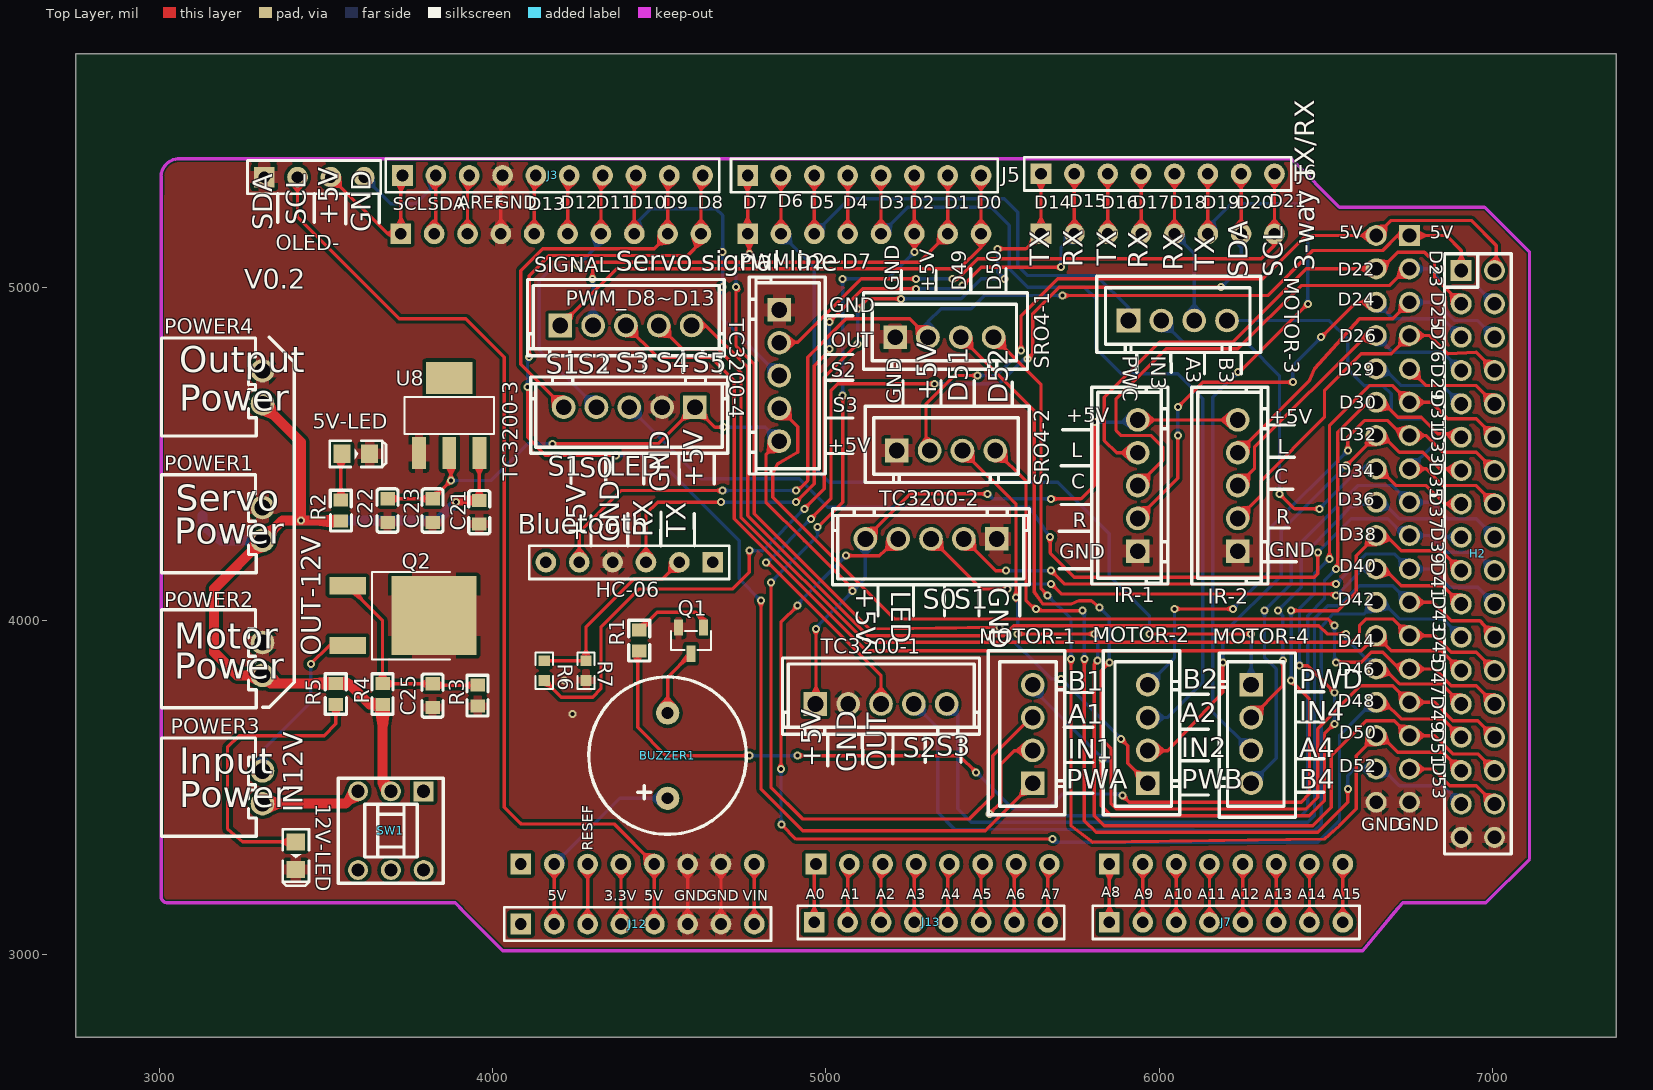
[diagram p0: Top Layer view]
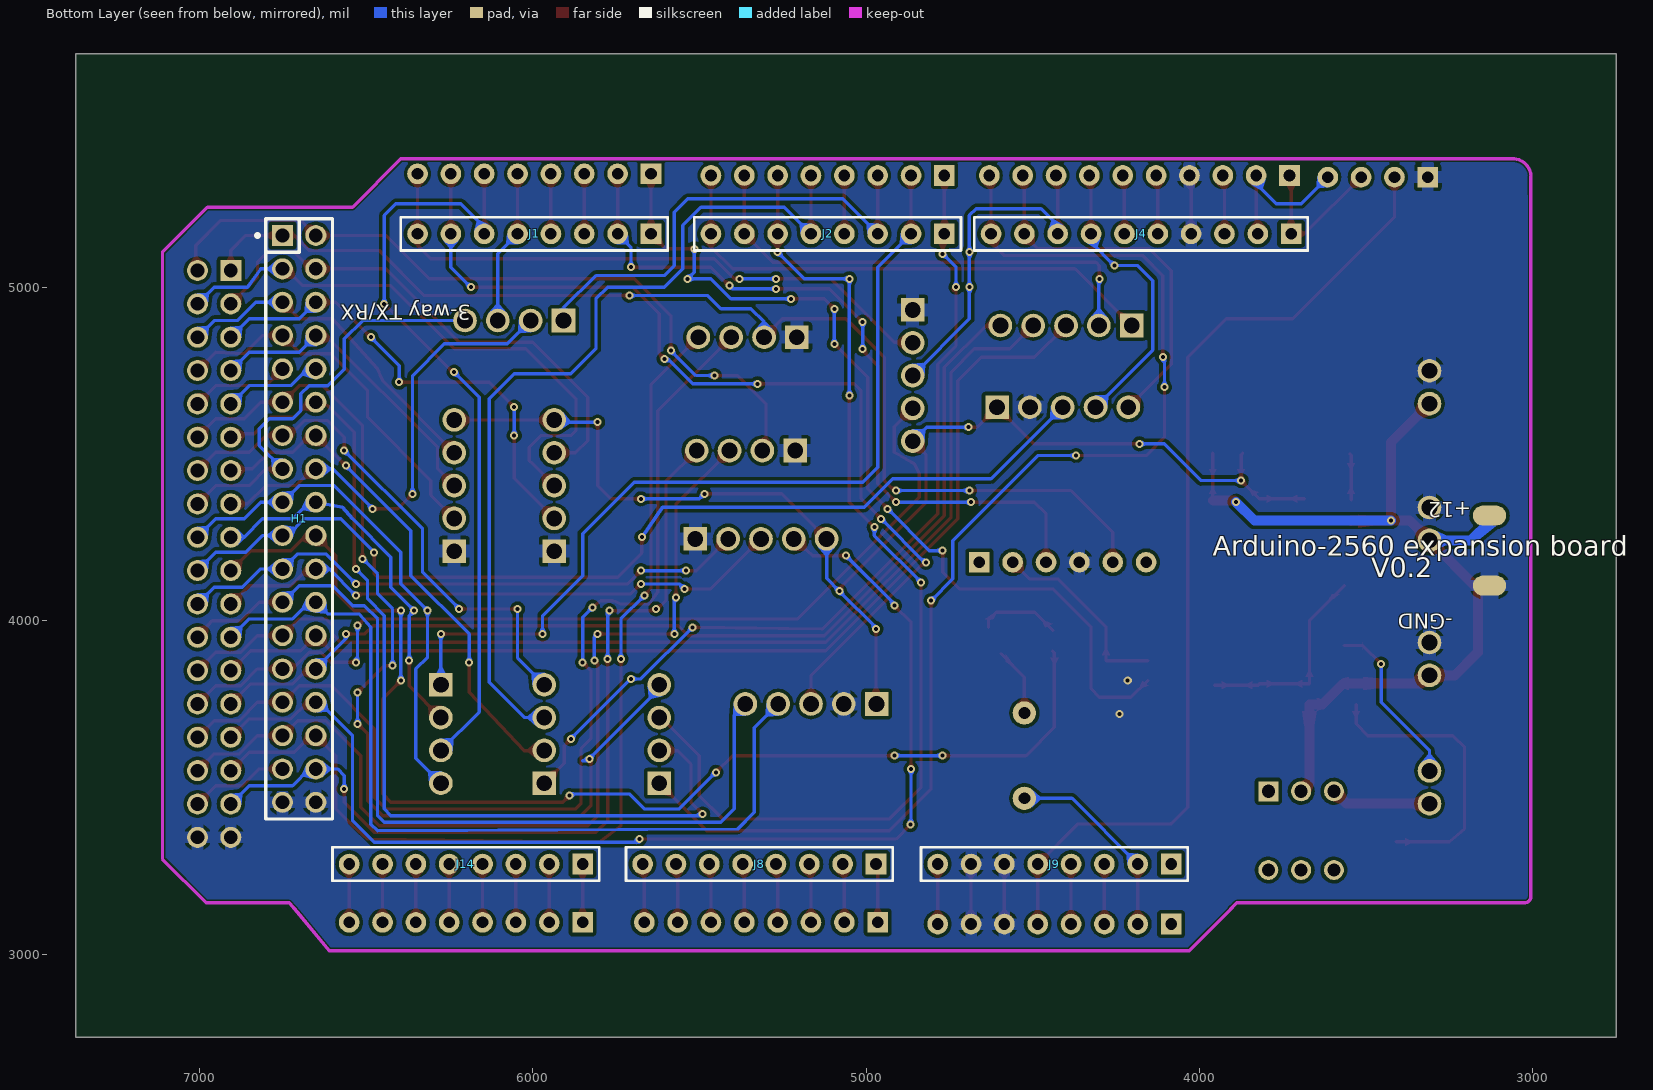
[diagram p1: Bottom Layer view, seen from below]
# Altium PCB MISC49934.pcbdoc (part 1 of 2)
Units mil, origin at the board's own origin, x right, y up, seen from the top; angles counter-clockwise.
Board outline 4620 x 2950 mil, 2 copper layers (Top Layer, Bottom Layer), stack 0 mil thick; 53 components, 145 nets, 295 pads, 118 vias.

## Layer stack, top to bottom
Top Layer: signal copper (thickness not stored)
Bottom Layer: signal copper (thickness not stored)

## Board outline
7370,2750 2750,2750 2750,5700 7370,5700

## Design rules (kind name [scope] priority, off if disabled: settings)
HoleToHoleClearance Default [All] p1 off: gap=0 allowstackedmicrovias=TRUE
HoleToHoleClearance gge14896 [All] p2 off: gap=0 allowstackedmicrovias=TRUE
HoleToHoleClearance gge14902 [All] p3 off: gap=0 allowstackedmicrovias=TRUE
HoleToHoleClearance Common [All] p4: gap=11.8 allowstackedmicrovias=TRUE

## Components (designator, comment, footprint, x,y, rotation, side; value= is the part's Value field where it differs from the comment)
5V-LED "LED-0805_R" LED0805_RED 3590,4500 r0 top
12V-LED "LED-0805_R" LED0805_RED 3410,3295 r270 top
+12 "Pad" 焊盘 3130,4315 r180 bottom
-GND "Pad" 焊盘 3130,4105 r180 bottom
BUZZER1 "GMC1205YA-16R2048" BUZ-TH_BD12.0-P6.50-D0.6-FD 4525,3595 r90 top
C21 "100nf" C0603 3960,4325 r90 top
C22 "100nf" C0603 3685,4330 r90 top
C23 "100nf" C0603 3820,4330 r90 top
C25 "100nf" C0603 3820,3775 r90 top
H1 "X6521WV-2×18H-C30D60" HDR-TH_36P-2.54-V-M-R2-C18-S2.54 6700,4305 r270 bottom locked
H2 "X6521WV-2×18H-C30D60" HDR-TH_36P-2.54-V-M-R2-C18-S2.54 6955,4200 r270 top locked
HC-06 "Bluetooth" HDR-F-2.54_1X6 4460,4175 r180 top
IR-1 "XH-5A_C722874" CONN-TH_XH-5A 5935,4405 r90 top
IR-2 "XH-5A_C722874" CONN-TH_XH-5A 6235,4405 r90 top
J1 "3-way TX/RX" HDR-M-2.54_1X8 6045,5160 r0 bottom locked
J2 "PWM D2~D7" HDR-M-2.54_1X8 5165,5160 r0 bottom locked
J3 "PWM_D8~D13" HDR-M-2.54_1X10#1 4180,5335 r0 top
J4 "PWM_D8~D13" HDR-M-2.54_1X10#2 4175,5160 r0 bottom
J5 "PWM D2~D7" HDR-M-2.54_1X8 5165,5335 r0 top
J6 "3-way TX/RX" HDR-M-2.54_1X8 6045,5340 r0 top
J7 "HDR-M-2.54_1x8" HDR-M-2.54_1X8 6250,3095 r0 top
J8 "HDR-M-2.54_1x8" HDR-M-2.54_1X8 5370,3270 r0 bottom
J9 "HDR-M-2.54_1x8" HDR-M-2.54_1X8 4485,3270 r0 bottom locked
J12 "HDR-M-2.54_1x8" HDR-M-2.54_1X8 4485,3090 r0 top
J13 "HDR-M-2.54_1x8" HDR-M-2.54_1X8 5365,3095 r0 top
J14 "HDR-M-2.54_1x8" HDR-M-2.54_1X8 6250,3270 r0 bottom locked
MOTOR-1 "MOTOR-1" CONN-TH_4P-P2.50_XH-4A 5620,3660 r90 top
MOTOR-2 "MOTOR-2" CONN-TH_4P-P2.50_XH-4A 5965,3660 r90 top
MOTOR-3 "MOTOR-3" CONN-TH_4P-P2.50_XH-4A 6055,4900 r0 top
MOTOR-4 "MOTOR-4" CONN-TH_4P-P2.50_XH-4A 6275,3660 r270 top
OLED- "OLED_" HDR-F-2.54_1X4 3465,5330 r0 top
POWER1 "XH-2AW" CONN-TH_2P-P2.50_XH-2AW 3310,4290 r90 top
POWER2 "XH-2AW" CONN-TH_2P-P2.50_XH-2AW 3310,3885 r90 top
POWER3 "XH-2AW" CONN-TH_2P-P2.50_XH-2AW 3310,3500 r90 top
POWER4 "XH-2AW" CONN-TH_2P-P2.50_XH-2AW 3310,4700 r90 top
Q1 "S8050" SOT-23-3_L2.9-W1.3-P1.90-LS2.4-BR 4595,3940 r90 top
Q2 "KIA50N03A" TO-252-2_L6.6-W6.1-P4.57-LS9.9-TL-CW 3695,4015 r0 top
R1 "10k" R0603#1 4440,3940 r90 top
R2 "200" R0603#1 3545,4330 r270 top
R3 "10K" R0603#1 3955,3775 r90 top
R4 "10k" R0603#1 3670,3780 r90 top
R5 "4.7k" R0603#1 3530,3780 r270 top
R6 "10K" R0603#2 4155,3850 r270 top
R7 "20K" R0603#2 4280,3850 r90 top
SIGNAL "XH-5A_C722874" CONN-TH_XH-5A 4400,4885 r0 top
SRO4-1 "Ultrasonic module" CONN-TH_4P-P2.50_XH-4A 5355,4850 r0 top
SRO4-2 "Ultrasonic module" CONN-TH_4P-P2.50_XH-4A 5360,4510 r0 top
SW1 "XKB8080-Z" SW-TH_6P-L8.0-W8.0-P2.50 3695,3370 r180 top
TC3200-1 "XH-5A_C722874" CONN-TH_XH-5A 5165,3750 r0 top
TC3200-2 "XH-5A_C722874" CONN-TH_XH-5A 5315,4245 r180 top
TC3200-3 "XH-5A_C722874" CONN-TH_XH-5A 4410,4640 r180 top
TC3200-4 "XH-5A_C722874" CONN-TH_XH-5A 4860,4735 r270 top
U8 "AMS1117-5.0" SOT-223_L6.5-W3.5-P2.30-LS7.0-BR 3870,4615 r270 top

## Footprints (in the part's own frame and the unit in brackets; to place one, negate y for a bottom-side part, rotate by r counter-clockwise, add the part's x,y. Pads: shape width x height; smd on the part's side, far side on the other; paste and mask are expansions set on the pad)
BUZ-TH_BD12.0-P6.50-D0.6-FD [mil]
  round 70 hole 35.4: 1(-128,0) 2(128,0)
  silkscreen extent -236,-236 236,236
C0603 [mm]
  rect 1x1.1 smd paste+0 mask+0.102: 1(-0.9,0) 2(0.9,0)
  silkscreen extent -1.65,-0.8 1.65,0.8
CONN-TH_2P-P2.50_XH-2AW [mm]
  round 1.8 hole 1.199: 1(-1.251,0) 2(1.251,0)
  silkscreen extent -3.71,0.48 3.75,7.7
CONN-TH_4P-P2.50_XH-4A [mm]
  rect 1.8x1.8 hole 1.199: 1(-3.75,0)
  round 1.8 hole 1.199: 2(-1.25,0) 3(1.25,0) 4(3.75,0)
  silkscreen extent -6.17,-2.44 6.33,3.38
CONN-TH_XH-5A [mm]
  rect 1.8x1.8 hole 1.2: 1(-5,0)
  round 1.8 hole 1.2: 2(-2.5,0) 3(0,0) 4(2.5,0) 5(5,0)
  silkscreen extent -7.5,-2.3 7.5,3.5
HDR-F-2.54_1X4 [mil]
  rect 62x62 hole 35: 1(-150,0)
  round 62 hole 35: 2(-50,0) 3(50,0) 4(150,0)
  silkscreen extent -200,-50 200,50
HDR-F-2.54_1X6 [mil]
  rect 62x62 hole 35: 1(-200,0)
  round 62 hole 35: 2(-100,0) 3(0,0) 4(100,0) 5(200,0) 6(300,0)
  silkscreen extent -250,-50 350,50
HDR-M-2.54_1X8 [mil]
  rect 62x62 hole 35: 1(-400,0)
  round 62 hole 35: 2(-300,0) 3(-200,0) 4(-100,0) 5(0,0) 6(100,0) 7(200,0) 8(300,0)
  silkscreen extent -450,-50 350,50
HDR-M-2.54_1X10#1 [mil]
  rect 62x62 hole 37.2: 1(-450,0)
  round 62 hole 35: 2(-350,0) 3(-250,0) 4(-150,0) 5(-50,0) 6(50,0) 7(150,0) 8(250,0) 9(350,0) 10(450,0)
  silkscreen extent -500,-50 500,50
HDR-M-2.54_1X10#2 [mil]
  rect 62x62 hole 35: 1(-450,0)
  round 62 hole 35: 2(-350,0) 3(-250,0) 4(-150,0) 5(-50,0) 6(50,0) 7(150,0) 8(250,0) 9(350,0) 10(450,0)
  silkscreen extent -500,-50 500,50
HDR-TH_36P-2.54-V-M-R2-C18-S2.54 [mm]
  rect 1.6x1.6 hole 1.05: 1(-21.59,-1.27)
  round 1.6 hole 1.05: 2(-21.59,1.27) 3(-19.05,-1.27) 4(-19.05,1.27) 5(-16.51,-1.27) 6(-16.51,1.27) 7(-13.97,-1.27) 8(-13.97,1.27) 9(-11.43,-1.27) 10(-11.43,1.27) 11(-8.89,-1.27) 12(-8.89,1.27) 13(-6.35,-1.27) 14(-6.35,1.27) 15(-3.81,-1.27) 16(-3.81,1.27) 17(-1.27,-1.27) 18(-1.27,1.27) 19(1.27,-1.27) 20(1.27,1.27) 21(3.81,-1.27) 22(3.81,1.27) 23(6.35,-1.27) 24(6.35,1.27) 25(8.89,-1.27) 26(8.89,1.27) 27(11.43,-1.27) 28(11.43,1.27) 29(13.97,-1.27) 30(13.97,1.27) 31(16.51,-1.27) 32(16.51,1.27) 33(19.05,-1.27) 34(19.05,1.27) 35(21.59,-1.27) 36(21.59,1.27)
  silkscreen extent -22.86,-3.3 22.86,2.54
LED0805_RED [mil]
  rect 51.2x55.1 smd: 1(-41.35,0) 2(41.35,0)
  silkscreen extent -79,-39 91,39
R0603#1 [mm]
  rect 1x1.1 smd paste+0 mask+0.102: 1(-0.8,0) 2(0.8,0)
  silkscreen extent -1.55,-0.8 1.55,0.81
R0603#2 [mm]
  rect 0.806x0.864 smd paste-100 mask+0.051: 1(-0.753,0) 2(0.753,0)
  silkscreen extent -1.39,-0.66 1.39,0.66
SOT-23-3_L2.9-W1.3-P1.90-LS2.4-BR [mm]
  rect 1.25x0.7 smd: 1(1,-0.95) 2(1,0.95) 3(-1,0)
  silkscreen extent -0.73,-1.53 0.73,1.53
SOT-223_L6.5-W3.5-P2.30-LS7.0-BR [mm]
  rect 2.465x1.05 smd: 1(2.858,-2.3) 2(2.857,0) 3(2.857,2.3)
  rect 2.465x3.54 smd: 4(-2.857,0)
  silkscreen extent -1.4,-3.4 1.4,3.4
SW-TH_6P-L8.0-W8.0-P2.50 [mil]
  rect 60x60 hole 39.37: 1(-98.41,-118.11)
  round 60 hole 39.37: 2(-0.01,-118.11) 3(98.41,-118.11) 4(-98.41,118.11) 5(-0.01,118.11) 6(98.41,118.11)
  silkscreen extent -157,-157 157,157
TO-252-2_L6.6-W6.1-P4.57-LS9.9-TL-CW [mm]
  rect 2.8x1.3 smd: 1(-3.292,2.273) 3(-3.292,-2.273)
  rect 6.5x6 smd: 2(3.292,0)
  silkscreen extent -1.46,-3.35 4.51,3.34
焊盘 [mil]
  oval 100x60 smd paste+0 mask+4: 1(0,0)

## Via types
v1: diameter 24, hole 12, Top Layer to Bottom Layer, 118 vias

## Nets (pads, with @x,y where several pads share a name; then routed paths per layer and width w, separated by ;. In a path a pad name is that pad's centre, name@x,y a point inside that pad or via, vN(x,y) a via of type N, cw(c..) or ccw(c..) an arc to the next point about the centre after c; other vN are vias at no path point)
3.3V: J9.4 J12.4 | length 180
  Top Layer w10: J12.4@4385,3090 J9.4@4385,3270
+5V_1: BUZZER1.1 J9.2 J12.2 | length 601.6
  Top Layer w10: J12.2@4185,3090 J9.2@4185,3270
  Bottom Layer w10: J9.2@4185,3270 4382,3467 BUZZER1.1@4525,3467
+5V_2: J9.5 J12.5 OLED-.2 | length 2964.7
  Top Layer w10: OLED-.2@3415,5330 3415,5210 3720,4905 3920,4905 4035,4790 4035,3440 4075,3400 4085.4,3390 ; 4085,3390 4365,3390 J9.5@4485,3270 J12.5@4485,3090
+5V_3: H1.1 H2.1 HC-06.5 SRO4-1.2 | length 3471.4
  Top Layer w10: HC-06.5@4260,4175 4260,4265 4385,4390 v1(4690,4390) ; v1(4910,4390) 4915,4390 4945,4420 4945,4790 5060,4905 5250.79,4905 SRO4-1.2@5305.79,4850 ; v1(5710,4975) 6325,4975 6460,5110 6670,5110 6715,5155 H1.1@6750,5155 6860,5155 6905,5110 H2.1@6905,5050
  Bottom Layer w10: v1(4690,4390) v1(4910,4390) ; SRO4-1.2@5305.79,4850 5305.79,4895.79 5345,4935 5435,4935 5475,4975 v1(5710,4975)
+5V_4: H1.2 H2.2 SRO4-2.2 | length 2251.9
  Top Layer w10: SRO4-2.2@5310.79,4510 5300,4520.79 5300,4550 5300,4650 5385,4735 v1(5455,4735) ; v1(5585,4810) 5585,4915 5695,5025 6310,5025 6440,5155 H1.2@6650,5155 6695,5200 6935,5200 7010,5125 7010,5055 H2.2@7005,5050
  Bottom Layer w10: v1(5455,4735) 5510,4735 v1(5585,4810)
_AREF: J3.3 J4.3 | length 177.1
  Top Layer w10: J4.3@3925,5160 3925,5330 J3.3@3930,5335
_SCL: J3.1 J4.1 OLED-.3 | length 457.5
  Top Layer w10: OLED-.3@3515,5330 3685,5160 J4.1@3725,5160 3725,5330 J3.1@3730,5335
_SDA: J3.2 J4.2 OLED-.4 | length 478
  Top Layer w10: J4.2@3825,5160 3830,5159.95 J3.2@3830,5335
  Bottom Layer w10: OLED-.4@3615,5330 3695,5250 3770,5250 3830,5310 J3.2@3830,5335
A0: J8.1 J13.1 | length 177.1
  Top Layer w10: J13.1@4965,3095 4965,3265 J8.1@4970,3270
A1: J8.2 J13.2 | length 177.1
  Top Layer w10: J13.2@5065,3095 5065,3265 J8.2@5070,3270
A2: J8.3 J13.3 | length 177.1
  Top Layer w10: J13.3@5165,3095 5165,3265 J8.3@5170,3270
A3: J8.4 J13.4 | length 177.1
  Top Layer w10: J13.4@5265,3095 5265,3265 J8.4@5270,3270
A4: J8.5 J13.5 | length 177.1
  Top Layer w10: J13.5@5365,3095 5365,3265 J8.5@5370,3270
A5: J8.6 J13.6 | length 177.1
  Top Layer w10: J13.6@5465,3095 5465,3265 J8.6@5470,3270
A6: J8.7 J13.7 | length 176.2
  Top Layer w10: J13.7@5565,3095 5565,3260 J8.7@5570,3270
A7: J8.8 J13.8 | length 177.1
  Top Layer w10: J13.8@5665,3095 5665,3265 J8.8@5670,3270
A8: J7.1 J14.1 | length 175
  Top Layer w10: J7.1@5850,3095 J14.1@5850,3270
A9: J7.2 J14.2 | length 175
  Top Layer w10: J7.2@5950,3095 J14.2@5950,3270
A10: J7.3 J14.3 | length 175
  Top Layer w10: J7.3@6050,3095 J14.3@6050,3270
A11: J7.4 J14.4 | length 175
  Top Layer w10: J7.4@6150,3095 J14.4@6150,3270
A12: J7.5 J14.5 | length 175
  Top Layer w10: J7.5@6250,3095 J14.5@6250,3270
A13: J7.6 J14.6 | length 175
  Top Layer w10: J7.6@6350,3095 J14.6@6350,3270
A14: J7.7 J14.7 | length 175
  Top Layer w10: J7.7@6450,3095 J14.7@6450,3270
A15: J7.8 J14.8 | length 175
  Top Layer w10: J7.8@6550,3095 J14.8@6550,3270
D0: J2.8 J5.8 SIGNAL.1 | length 1574.2
  Top Layer w10: SIGNAL.1@4203.1,4885 4373.1,5055 5400,5055 5465,5120 J2.8@5465,5160 J5.8@5465,5335
D1: J2.7 J5.7 SIGNAL.2 | length 1460
  Top Layer w10: v1(4300,5025) 4300,5065 4310,5075 5280,5075 J2.7@5365,5160 J5.7@5365,5335
  Bottom Layer w10: v1(4300,5025) 4301.58,5023.42 SIGNAL.2@4301.58,4885.01
D2: J2.6 J5.6 MOTOR-1.3 | length 3439.4
  Top Layer w10: v1@4835,4120 4835,3500 4930,3405 5430,3405 5500,3475 5500,3594.2 MOTOR-1.3@5620,3714.2 ; v1(4975,4280) 5050,4355 ; v1(5265,5105) J2.6@5265,5160 J5.6@5265,5335 ; 5050,4355 v1(5050,4675) 5050,4355
  Bottom Layer w10: v1(4835,4115) 4975,4255 v1(4975,4280) ; v1(5050,4675) v1(5050,5025) 5185,5025 v1(5265,5105)
D3: J2.5 J5.5 MOTOR-2.3 | length 2634.1
  Top Layer w10: J2.5@5165,5160 J5.5@5165,5335
  Bottom Layer w10: J2.5@5165,5160 5245,5240 5495,5240 5550,5185 5550,5055 5605,5000 5775,5000 5810,4965 5810,4815 5885,4740 6055,4740 6130,4665 6130,3815 6024.21,3709.21 MOTOR-2.3@5965,3709.21
D4: J2.4 J5.4 | length 175
  Top Layer w10: J2.4@5065,5160 J5.4@5065,5335
D5: J2.3 J5.3 MOTOR-3.1 | length 1427.8
  Top Layer w10: J2.3@4965,5160 J5.3@4965,5335
  Bottom Layer w10: J2.3@4965,5160 5070,5265 5535,5265 5575,5225 5575,5065 5605,5035 5810,5035 5907.3,4937.6 MOTOR-3.1@5907.3,4900
D6: J2.2 J5.2 MOTOR-4.1 | length 2691.4
  Top Layer w10: J2.2@4865,5160 J5.2@4865,5335 ; v1(5970,3960) v1(6275,3960)
  Bottom Layer w10: J2.2@4865,5160 4965,5060 4965,4460 5010,4415 5695,4415 5850,4260 5850,4135 5970,4015 v1(5970,3960) ; MOTOR-4.1@6275,3807.65 v1(6275,3960)
D7: J2.1 J5.1 MOTOR-2.1 | length 2603.4
  Top Layer w10: v1(4730,5000) 4730,4825 4785,4768.4 4785,4320 5130,3975 5135,3975 v1(5520,3980) ; J5.1@4765,5335 J2.1@4765,5160 4770,5155 v1(4770,5100) ; v1(5885,3645) 5905,3625 5905,3572.4 MOTOR-2.1@5965,3512.35
  Bottom Layer w10: v1(4730,5000) 4730,5060 v1(4770,5100) ; v1(5520,3980) 5675,3825 v1(5705,3825) v1(5885,3645)
D8: J3.10 J4.10 MOTOR-1.1 | length 3706.7
  Top Layer w10: v1(4105,4700) 4105,4550 4160,4495 v1(4370,4495) ; v1(4110,4790) 4110,5035 4170,5095 4585,5095 4625,5135 J4.10@4625,5160 4625,5330 J3.10@4630,5335 ; v1(4805,4060) 4805,3495 4930,3370 5435,3370 5477.7,3370 MOTOR-1.1@5620,3512.35
  Bottom Layer w10: v1(4105,4700) 4105,4785 v1(4110,4790) ; v1(4370,4495) 4485,4495 4740,4240 4740,4125 v1(4805,4060)
D9: J3.9 J4.9 TC3200-3.5 | length 1128.6
  Top Layer w10: TC3200-3.5@4213.1,4640 4085,4768.2 4085,5050 4150,5115 4485,5115 4525,5155 J4.9@4525,5160 4525,5330 J3.9@4530,5335
D10: J3.8 J4.8 TC3200-4.3 | length 1046.5
  Top Layer w10: J4.8@4425,5160 4425,5330 J3.8@4430,5335
  Bottom Layer w10: J4.8@4425,5160 4425,5185 4475,5235 4670,5235 4690,5215 v1(4690,5105) v1(4690,5000) 4690,4905 TC3200-4.3@4860,4735
D11: J3.7 J4.7 TC3200-3.4 | length 885.8
  Top Layer w10: J4.7@4325,5160 4325,5330 J3.7@4330,5335
  Bottom Layer w10: TC3200-3.4@4311.57,4639.99 4140,4811.57 4140,5020 4185,5065 v1(4255,5065) 4325,5135 J4.7@4325,5160
D12: J3.6 J4.6 | length 177.1
  Top Layer w10: J4.6@4225,5160 4225,5330 J3.6@4230,5335
D13: J3.5 J4.5 | length 177.1
  Top Layer w10: J4.5@4125,5160 4125,5330 J3.5@4130,5335
D14: J1.1 J6.1 R6.2 | length 3580.6
  Top Layer w10: v1(4770,4210) 4770,4145 4720,4095 ; v1(4935,4335) 4995,4395 4995,4730 v1(5095,4830) ; v1(5095,4935) 5125,4965 v1(5225,4965) ; v1(5515,5115) 5600,5115 J1.1@5645,5160 J6.1@5645,5340 ; 4205.3,3770 R6.2@4155,3820.34 4205.3,3770 ; 4205.3,3770 4300,3770 ; 4205.3,3770 4300,3770 ; 4300,3770 4325,3795 ; 4300,3770 4325,3795 ; 4325,3795 4325,3980 ; 4325,3795 4325,3980 ; 4325,3980 4440,4095 ; 4325,3980 4440,4095 ; 4440,4095 4720,4095 ; 4440,4095 4720,4095
  Bottom Layer w10: v1(4770,4210) 4810,4210 v1(4935,4335) ; v1(5095,4830) v1(5095,4935) ; v1(5225,4965) 5405,4965 5465,5025 v1(5535,5025) 5515,5045 v1(5515,5115)
  other v1: 5095,4935
D15: HC-06.3 J1.2 J6.2 | length 2250.8
  Top Layer w10: HC-06.3@4460,4175 4460,4320 4495,4355 v1(4685,4355) ; v1(4910,4355) 4965,4410 4965,4765 5010,4810 v1(5010,4815) ; v1(5010,4895) 5110,4995 v1(5270,4995) ; v1(5410,5005) 5465,5060 v1(5705,5060) ; J1.2@5745,5160 J6.2@5745,5340
  Bottom Layer w10: v1(4685,4355) v1(4910,4355) ; v1(5010,4815) v1(5010,4895) ; v1(5270,4995) 5400,4995 v1(5410,5005) ; v1(5705,5060) 5705,5120 J1.2@5745,5160
D16: J1.3 J6.3 | length 180
  Top Layer w10: J1.3@5845,5160 J6.3@5845,5340
D17: J1.4 J6.4 | length 180
  Top Layer w10: J1.4@5945,5160 J6.4@5945,5340
D18: J1.5 J6.5 MOTOR-3.3 | length 464.5
  Top Layer w10: J1.5@6045,5160 J6.5@6045,5340
  Bottom Layer w10: J1.5@6045,5160 6104.21,5100.79 MOTOR-3.3@6104.21,4900
D19: J1.6 J6.6 MOTOR-4.3 | length 2323.4
  Top Layer w10: J1.6@6145,5160 J6.6@6145,5340 ; v1(6235,4745) 6240,4745 v1(6445,4950) v1@6450,4955
  Bottom Layer w10: J1.6@6145,5160 6145,5180 6215,5250 6410,5250 6440,5220 6445,5215 v1(6445,4950) ; v1(6235,4745) 6160,4670 6160,4555.27 6160,3725.79 MOTOR-4.3@6275,3610.79
D20: J1.7 J6.7 TC3200-1.3 | length 3560.2
  Top Layer w10: v1(4820,4175) 4825,4175 5165,3835 TC3200-1.3@5165,3750 ; v1(5325,4710) 5035,4710 5015,4690 ; 5695,4995 5620,4920 ; v1(6185,5000) 5700,5000 5620,4920 ; J1.7@6245,5160 J6.7@6245,5340 ; 5015,4365 v1(4955,4305) 5015,4365 ; 5015,4365 5015,4690 ; 5015,4365 5015,4670 5015,4690 ; 5620,4800 v1(5605,4785) 5620,4800 ; 5620,4800 5620,4920 ; 5620,4800 5620,4920
  Bottom Layer w10: v1(4820,4175) 4825,4175 v1(4955,4305) ; v1(5325,4710) 5520,4710 5595,4785 v1(5605,4785) ; v1(6185,5000) 6245,5060 J1.7@6245,5160
D21: J1.8 J6.8 TC3200-4.2 | length 1899.3
  Top Layer w10: TC3200-4.2@4860.01,4833.42 4861.58,4835 4915,4835 5105,5025 v1(5270,5025) ; v1(5380,5025) 5395,5025 5455,5085 6305,5085 6345,5125 J1.8@6345,5160 J6.8@6345,5340
  Bottom Layer w10: v1@5267.5,5025 v1@5372.5,5025 ; v1(5270,5025) 5350,5025 5353.57,5025
D22: H1.4 H2.3 IR-1.4 | length 1585.9
  Top Layer w10: IR-1.4@5934.99,4503.43 5871.6,4503.4 5835,4540 5835,4670 6000,4835 6220,4835 6440,5055 H1.4@6650,5055 6665,5055 6715,5105 6795,5105 6825,5075 6825,5030 H2.3@6905,4950
D23: H1.3 H2.4 IR-1.3 | length 1747
  Top Layer w10: IR-1.3@5935,4405 6000,4470 6010,4480 6010,4520 5975,4555 5885,4555 5870,4570 5870,4665 6020,4815 6235,4815 6425,5005 6690,5005 6740,5055 H1.3@6750,5055
  Bottom Layer w10: H1.3@6750,5055 6815,5055 6855,5000 6955,5000 H2.4@7005,4950
D24: H1.6 H2.5 IR-1.2 | length 1436.4
  Top Layer w10: IR-1.2@5934.99,4306.58 6055,4426.58 v1(6055,4555) ; v1(6055,4640) 6130,4715 v1(6400,4715) ; v1(6485,4850) 6590,4955 H1.6@6650,4955
  Bottom Layer w10: v1(6055,4555) v1(6055,4640) ; v1(6400,4715) 6400,4765 v1(6485,4850) ; H1.6@6650,4955 6700,4905 6850,4905 H2.5@6905,4850
D25: H1.5 H2.6 IR-2.4 | length 1014.3
  Top Layer w10: IR-2.4@6234.99,4503.43 6450,4720 6465,4755 6600,4905 6700,4905 H1.5@6750,4955
  Bottom Layer w10: H1.5@6750,4955 6830,4955 6885,4900 6955,4900 H2.6@7005,4850
D26: H1.8 H2.7 IR-2.3 | length 963
  Top Layer w10: IR-2.3@6235,4430 IR-2.3@6235,4405 6285,4455 6285,4520 6620,4855 H1.8@6650,4855
  Bottom Layer w10: H1.8@6650,4855 6700,4805 6850,4805 H2.7@6905,4750
D27: H1.7 H2.8 IR-2.2 | length 1115.2
  Top Layer w10: IR-2.2@6234.99,4306.58 6305,4376.6 6305,4420 6495,4610 6495,4690 6605,4800 6695,4800 H1.7@6750,4855 6810,4855 6865,4800 6950,4805 6960,4795 H2.8@7005,4750
D28: H1.10 H2.9 | length 298.5
  Bottom Layer w10: H1.10@6650,4755 6675,4755 6725,4705 6850,4705 H2.9@6905,4650
D29: H1.9 H2.10 | length 298.5
  Top Layer w10: H1.9@6750,4755 6800,4705 6950,4705 H2.10@7005,4650
D30: H1.12 H2.11 MOTOR-1.2 | length 2857.1
  Top Layer w10: v1(5490,3420) 5525,3455 5525,3570 5565,3610 5619.21,3610 MOTOR-1.2@5620,3610.79 ; v1(6530,4155) 6535,4160 6535,4565 6600,4630 6615,4645 H1.12@6650,4655 6670,4655 6715,4610 6785,4610 6835,4560 6895,4560 H2.11@6905,4550
  Bottom Layer w10: v1(5490,3420) 5495,3415 6425,3415 6445,3435 6445,4015 6495,4065 6495,4120 v1(6530,4155)
D31: H1.11 H2.12 MOTOR-1.4 | length 3016.6
  Top Layer w10: v1(5830,3585) 5825,3580 5825,3445 5855,3415 6450,3415 6495,3460 6495,3660 v1(6525,3690) ; v1(6420,3865) 6445,3865 v1(6525,3785) ; v1(6510,4185) 6510,4585 6630,4705 6700,4705 H1.11@6750,4655 6815,4655 6865,4605 6950,4605 H2.12@7005,4550
  Bottom Layer w10: MOTOR-1.4@5620,3807.65 5620,3795 v1(5830,3585) 5835,3580 5850,3580 ; v1(6420,3865) 6420,4035 6465,4080 6465,4140 v1(6510,4185) ; v1(6525,3690) v1(6525,3785)
D32: H1.14 H2.13 MOTOR-2.2 | length 1559.9
  Top Layer w10: MOTOR-2.2@5965,3610.79 5965.79,3610 6025,3610 6190,3785 v1(6190,3875) ; v1(6560,4465) H1.14@6650,4555 6670,4555 6720,4505 6790,4505 6840,4455 6900,4455 H2.13@6905,4450
  Bottom Layer w10: v1(6190,3875) 6190,3960 6365,4135 6365,4270 v1(6560,4465)
D33: H1.13 H2.14 MOTOR-2.4 | length 1616.2
  Top Layer w10: v1(6045,4035) v1(6220,4035) ; v1(6565,4510) 6565,4550 6615,4600 6685,4600 6730,4555 H1.13@6750,4555 6800,4555 6850,4505 6950,4505 H2.14@7005,4450
  Bottom Layer w10: MOTOR-2.4@5965,3807.65 6045,3887.65 v1(6045,4035) ; v1(6220,4035) 6330,4145 6330,4275 v1(6565,4510)
D34: H1.16 H2.15 MOTOR-3.2 | length 2101.9
  Top Layer w10: v1(6360,4380) 6405,4335 v1(6480,4335) ; H1.16@6650,4455 6660,4455 6710,4405 6800,4405 6855,4350 H2.15@6905,4350
  Bottom Layer w10: v1(6360,4380) 6360,4490 ; v1(6480,4335) 6600,4455 H1.16@6650,4455 ; 6075.79,4830 MOTOR-3.2@6005.79,4900 6075.79,4830 ; 6075.79,4830 6265,4830 ; 6075.79,4830 6265,4830 ; 6265,4830 6360,4735 ; 6265,4830 6360,4735 ; 6360,4490 6360,4735 ; 6360,4490 6360,4735
D35: H1.15 H2.16 MOTOR-3.4 | length 1282.2
  Top Layer w10: H1.15@6750,4455 6800,4455 6850,4405 6950,4405 H2.16@7005,4350
  Bottom Layer w10: MOTOR-3.4@6202.7,4900 6510,4900 6565,4845 6565,4753.64 6614.01,4704.62 6670.38,4704.62 6695,4680 6695,4630 6720,4605 6790,4605 6820,4575 6820,4525 H1.15@6750,4455
D36: H1.18 H2.17 MOTOR-4.2 | length 1144
  Top Layer w10: MOTOR-4.2@6275,3709.21 6370,3804.21 v1(6370,3880)
  Bottom Layer w10: v1(6370,3880) 6370,4015 v1(6355,4030) 6425,4100 6425,4190 6540,4305 6570,4340 H1.18@6650,4355 6670,4355 6720,4305 6810,4305 6865,4250 H2.17@6905,4250
D37: H1.17 H2.18 MOTOR-4.4 | length 1882.1
  Bottom Layer w10: 6350,3835 6350,3587.35 ; H2.18@7005,4250 6950,4305 6865,4305 6815,4355 H1.17@6750,4355 6700,4405 6595,4405 6395,4205 6395,4110 v1(6315,4030) 6315,3890 6350,3855 6350,3587.35 ; 6350,3587.35 MOTOR-4.4@6275,3512.35 6350,3587.35
D38: H1.20 H2.19 R1.1 | length 3711.9
  Top Layer w10: R1.1@4440,3908.51 4435,3903.5 4435,3680 4520,3595 v1(4770,3595) ; v1(4915,3595) 5400,3595 v1(5450,3545) ; v1(5890,3475) 5910,3455 6425,3455 6450,3480 6450,3765 v1(6395,3820) ; v1(6395,4030) 6535,4030 6590,4085 6590,4195 ; 6590,4163.43 6590,4195 ; 6590,4185 6590,4190 6590,4195 ; H2.19@6905,4150 6845,4210 6725,4210 6680,4255 H1.20@6650,4255 6590,4195
  Bottom Layer w10: v1(4770,3595) v1(4915,3595) ; v1(5450,3545) 5560,3435 5665,3435 5710,3480 5885,3480 v1(5890,3475) ; v1(6395,3820) v1(6395,4030)
D39: H1.19 H2.20 TC3200-3.3 | length 3018.6
  Top Layer w10: v1(5672.29,4250.03) 5672.3,4202.7 5745,4130 6465,4130 6475,4140 v1(6474.9,4204.9)
  Bottom Layer w10: TC3200-3.3@4410,4640 4625,4425 4920,4425 5005,4340 5610,4340 v1(5672.29,4250.03) ; v1(6474.9,4204.9) 6575,4305 6685,4305 6735,4255 H1.19@6750,4255 6810,4255 6821.1,4243.9 6860,4205 6950,4205 H2.20@7005,4150
D40: H1.22 H2.21 TC3200-2.3 | length 1752.4
  Top Layer w10: TC3200-2.3@5315,4245 5465,4095 v1(5545,4095) ; v1(5675,4110) 5705,4080 6530,4080 v1(6530,4075) ; H1.22@6650,4155 6675,4155 6725,4105 6850,4105 H2.21@6905,4050
  Bottom Layer w10: v1(5545,4095) 5560,4110 v1(5675,4110) ; v1(6530,4075) 6610,4155 H1.22@6650,4155
D41: H1.21 H2.22 TC3200-2.2 | length 1746.9
  Top Layer w10: TC3200-2.2@5413.42,4244.99 5508.42,4150 v1(5540,4150) ; v1(5675,4150) 5715,4110 v1(6530,4110)
  Bottom Layer w10: v1(5540,4150) v1(5675,4150) ; v1(6530,4110) 6620,4200 6705,4200 H1.21@6750,4155 6815,4155 6870,4100 6955,4100 6970,4085 H2.22@7005,4050
  other v1: 5675,4150
D42: H1.24 H2.23 TC3200-1.4 | length 2634
  Bottom Layer w10: TC3200-1.4@5263.43,3750.01 5335,3678.4 5335,3425 5385,3375 6465,3370 6485,3389.3 6485,3980 6520,4020 ; 6534,4020 6520,4020 ; H2.23@6905,3950 6850,4005 6720,4005 6670,4055 H1.24@6650,4055 6615,4020 6520,4020
D43: H1.23 H2.24 TC3200-1.5 | length 2666.4
  Top Layer w10: H1.23@6750,4055 6820,4055 6875,4000 6961.3,4000 H2.24@7005,3950
  Bottom Layer w10: TC3200-1.5@5361.9,3750 5395,3716.8 5395,3435 5435,3395 6445,3395 6465,3415 6465,4005 6505,4045 6530.2,4045 ; 6525,4045 6540,4045 6600,4105 6700,4105 H1.23@6750,4055
D44: H1.26 H2.25 SIGNAL.3 | length 3214.2
  Top Layer w10: SIGNAL.3@4400,4885 4495,4790 4655,4790 4725,4720 4725,4305 5120,3910 6605.4,3910 H1.26@6650,3955 6695,3910 6845,3910 H2.25@6905,3850
D45: H1.25 H2.26 SIGNAL.4 | length 3263.6
  Top Layer w10: SIGNAL.4@4498.43,4885.01 4568.4,4815 4675,4815 4745,4745 4745,4310 5120,3935 6576.44,3935 6600,3958.56 6600,3985 6620,4005 6700,4005 H1.25@6750,3955 6825,3955 6875,3905 6950,3905 H2.26@7005,3850
D46: H1.28 H2.27 SIGNAL.5 | length 3072.5
  Top Layer w10: SIGNAL.5@4596.9,4885 4640,4885 4765,4760 4765,4315 5125,3955 5533.6,3955 5563.6,3985 6478.4,3985 6503.4,3960 v1(6560,3960) ; H1.28@6650,3855 6675,3855 6720,3810 6845,3810 H2.27@6905,3750
  Bottom Layer w10: v1(6560,3960) 6560,3945 H1.28@6650,3855
D47: H1.27 H2.28 TC3200-4.4 | length 2835.6
  Top Layer w10: TC3200-4.4@4860.01,4636.57 4915,4581.6 4915,4505 4855,4470 4840,4440 4840,4370 5205,4005 6505,4005 v1(6525,3985) ; v1(6530,3875) 6605,3875 6635,3905 6670,3905 6710,3865 6740,3865 H1.27@6750,3855 6825,3855 6875,3805 6950,3805 H2.28@7005,3750
  Bottom Layer w10: v1(6525,3985) 6525,3880 v1(6530,3875)
D48: H1.30 H2.29 TC3200-2.4 | length 3522.5
  Top Layer w10: v1(4865,3555) 4865,3995 v1(4915,4045) ; v1(4866.95,3388.05) 4910,3345 v1(5680,3345) ; v1(5060,4195) 5155,4195 5160,4195 5215,4245 TC3200-2.4@5216.57,4244.99 ; H1.30@6650,3755 6675,3755 6725,3705 6850,3705 H2.29@6905,3650
  Bottom Layer w10: v1(4865,3555) 4865,3390 v1(4866.95,3388.05) ; v1(4915,4045) 4915,4050 v1(5060,4195) ; v1@5680,3335 6475,3335 6540,3400 6540,3655 6600,3715 ; 6575,3690 6640,3755 H1.30@6650,3755
D49: H1.29 H2.30 SRO4-1.3 | length 3198.1
  Top Layer w10: SRO4-1.3@5404.21,4850 5625,4629.2 5625,4085 5650,4050 5735,4050 5760,4060 5795,4060 v1(5820,4040) ; v1(5850,3875) 5825,3850 5825,3645 5855,3615 5855,3450 5870,3435 6440,3435 6475,3470 6475,3675 6602.6,3805 6700,3805 H1.29@6750,3755 6825,3755 6880,3700 6955,3700 H2.30@7005,3650
  Bottom Layer w10: v1(5820,4040) 5850,4010 v1(5850,3875)
D50: H1.32 H2.31 SRO4-1.4 | length 3012.6
  Top Layer w10: SRO4-1.4@5502.65,4850 5645,4707.65 5645,4095 v1(5665,4075) ; v1(5735,3885) 5735,3385 5800,3335 6495,3345 6540,3385 6590,3435 6590,3595 H1.32@6650,3655 6665,3655 6715,3605 6850,3605 H2.31@6905,3550
  Bottom Layer w10: v1(5665,4075) 5735,4005 v1(5735,3885)
D51: H1.31 H2.32 SRO4-2.3 | length 3414.4
  Top Layer w10: v1@5570,4060 5570,4349.21 ; v1(5570,4070) 5570,4349.21 ; v1(5575,3960) v1(5805,3960) ; v1(5815,3880) 5805,3870 5805,3415 5835,3385 6460,3385 6515,3440 6515,3595 6620,3700 6705,3700 H1.31@6750,3655 6825,3655 6880,3600 6955,3600 H2.32@7005,3550 ; 5570,4349.21 SRO4-2.3@5409.21,4510 5570,4349.21
  Bottom Layer w10: v1(5570,4070) 5575,4065 v1(5575,3960) ; v1(5805,3960) 5815,3950 v1(5815,3880)
D52: H1.34 H2.33 SRO4-2.4 | length 3907.7
  Top Layer w10: SRO4-2.4@5507.65,4510 5600,4417.65 5600,4060 5625,4035 v1(5630,4035) 5635,4030 v1(5770,4030) ; 6540,3430 6530,3420 6475,3365 ; v1(6565,3495) 6565,3455 6475,3365 ; 5775,3400 v1(5775,3885) 5775,3400 ; 5775,3400 5810,3365 ; 5775,3400 5810,3365 ; 5810,3365 6475,3365 ; 5810,3365 6475,3365
  Bottom Layer w10: v1(5770,4030) 5775,4025 v1(5775,3885) ; v1(6565,3495) 6565,3535 6585,3555 H1.34@6650,3555 6670,3555 6720,3505 6850,3505 H2.33@6905,3450
D53: H1.33 H2.34 | length 298.5
  Top Layer w10: H1.33@6750,3555 6820,3555 6870,3505 6950,3505 H2.34@7005,3450
GND: 5V-LED.2 12V-LED.2 -GND.1 C21.1 C22.1 C23.1 C25.1 H1.35 H1.36 H2.35 H2.36 HC-06.4 IR-1.1 IR-2.1 J3.4 J4.4 J9.6 J9.7 J12.6 J12.7 OLED-.1 POWER1.2 POWER2.2 POWER4.2 Q1.2 Q2.2 R3.1 R7.1 SRO4-1.1 SRO4-2.1 TC3200-1.2 TC3200-2.1 TC3200-3.2 TC3200-4.1 U8.1 | length 537.1
  Top Layer w10: J4.4@4025,5160 4025,5330 J3.4@4030,5335 ; J12.6@4585,3090 J9.6@4585,3270 ; J12.7@4685,3090 J9.7@4685,3270
  other v1: 4240,3720 4215,3820
HC-06_2: HC-06.2 R6.1 R7.2 | length 586.1
  Top Layer w10: R6.1@4155,3879.66 R7.2@4280,3879.66 ; R7.2@4280,3879.66 4280,3980 4425,4125 4510,4125 HC-06.2@4560,4175
OUT1_+5V: C22.2 C23.2 IR-1.5 IR-2.5 TC3200-1.1 TC3200-2.5 TC3200-3.1 TC3200-4.5 U8.2 | length 3990.9
  Top Layer w10: C22.2@3685,4365.44 C23.2@3820,4365.44 3874.6,4420 v1(3875,4420) 3875,4497.5 U8.2@3870,4502.5 ; v1(4180,4530) 4496.85,4530 TC3200-3.1@4606.85,4640 ; TC3200-3.1@4606.9,4640 4666.9,4580 v1@4700,4580 ; TC3200-4.5@4860,4538.1 4820,4498.1 4820,4355 4934.7,4240.3 4935,4240 ; 4930,4245 5080,4095 v1(5080,4088.53) ; TC3200-1.1@4968.1,3750 4970,3751.9 v1(4970,3975) ; TC3200-2.5@5118.15,4245 5253.15,4380 v1(5485,4380) ; v1(5675,4365) 5765,4365 5805,4405 v1(5805,4595) ; IR-1.5@5935,4601.85 IR-2.5@6235,4601.85
  Bottom Layer w10: v1(3875,4420) 3995,4420 4105,4530 v1(4180,4530) ; v1(4692.22,4580) 4818.2,4580 TC3200-4.5@4860,4538.15 ; v1(4970,3975) 4970,3978.53 v1(5080,4088.53) 5118.15,4126.68 TC3200-2.5@5118.15,4245 ; 5520,4365 5500,4365 ; v1(5675,4365) 5500,4365 ; v1(5805,4595) 5928.15,4595 IR-1.5@5935,4601.85 ; 5500,4365 v1(5485,4380) 5500,4365
Q1_1: Q1.1 R1.2 | length 247
  Top Layer w10: R1.2@4440,3971.5 4493.5,4025 4610,4025 4632.4,4002.6 Q1.1@4632.4,3979.37
Q1_3: BUZZER1.2 Q1.3 | length 206.6
  Top Layer w10: BUZZER1.2@4525,3723 4525,3830.6 Q1.3@4595,3900.63
Q2_1: C25.2 Q2.1 R3.2 R4.2 | length 623.4
  Top Layer w10: Q2.1@3565.4,4104.48 3670,3999.9 R4.2@3670,3811.5 3671.1,3810.4 C25.2@3820,3810.44 3823.9,3806.5 R3.2@3955,3806.5
Q2_3: POWER3.2 Q2.3 | length 514.2
  Top Layer w10: v1(3455,3870) 3510,3925 Q2.3@3565.4,3925.52
  Bottom Layer w10: POWER3.2@3310,3549 3310,3610 3455,3755 v1(3455,3870)
R2_1: 5V-LED.1 R2.1 | length 140
  Top Layer w10: R2.1@3545,4361.49 3545,4496.4 5V-LED.1@3548.65,4500
R5_2: 12V-LED.1 R5.2 | length 876.8
  Top Layer w10: 12V-LED.1@3410,3336.35 3250,3336.4 3205,3375 3205,3620 3240,3655 3495,3655 3530,3690 R5.2@3530,3748.5
RESEF: J9.3 J12.3 | length 180
  Top Layer w10: J12.3@4285,3090 J9.3@4285,3270
S$3075: 
S$3942: 
S$3947: 
S$3949: 
S$3952: 
S$3954: 
S$3958: 
S$3961: 
S$3963: 
S$3965: 
S$3975: 
S$3977: 
S$11567: 
S$11623: 
S$12201: 
S$12203: 
S$12205: 
S$12209: 
S$12241: 
S$12243: 
S$12245: 
S$12247: 
S$12361: 
S$12363: 
S$12365: 
S$12369: 
S$12371: 
S$12373: 
S$12375: 
S$12377: 
S$12379: 
S$12417: 
S$12419: 
S$12421: 
S$12423: 
S$12425: 
S$12427: 
S$12429: 
S$12431: 
S$12433: 
S$12435: 
S$12437: 
S$12583: 
S$12586: 
S$12588: 
S$12590: 
S$12592: 
S$12594: 
S$12596: 
S$12598: 
S$12601: 
S$12603: 
S$14301: 
S$14520: 
SW1_3: POWER3.1 SW1.3 | length 302.1
  Top Layer w30: POWER3.1@3310,3450.75 3559.25,3450.75 SW1.3@3596.59,3488.11